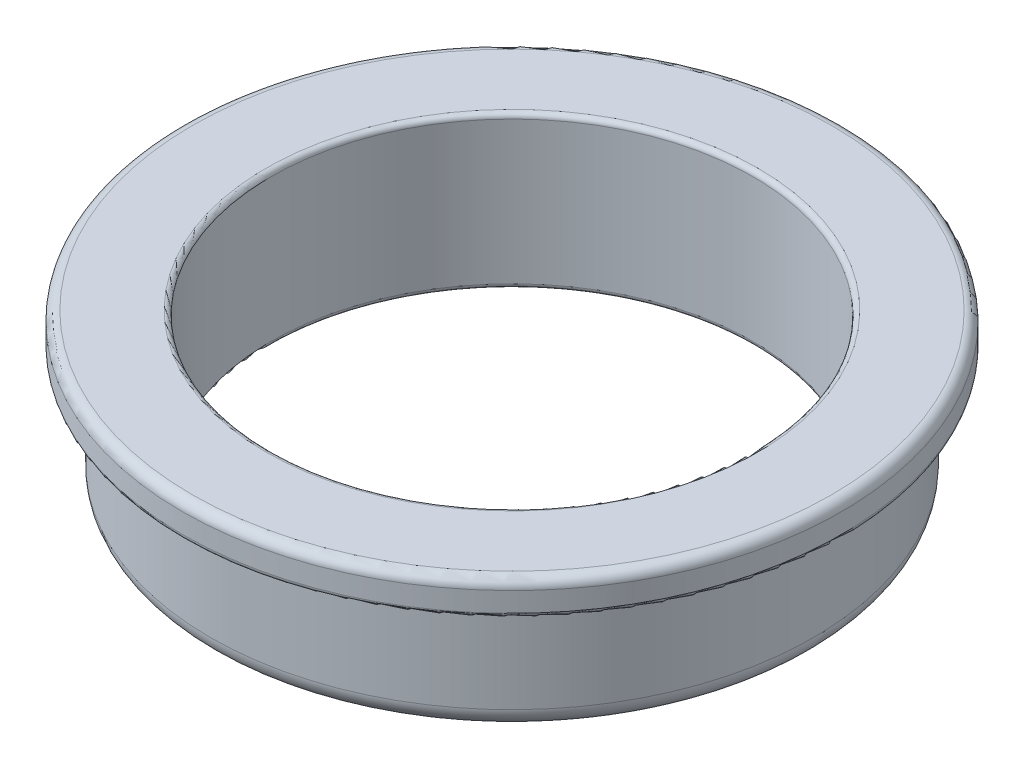
SolidWorks part; units mm, degrees
material "S45C"
ref_plane "Front Plane" through (0, 0, 0) normal (0, 0, 1) x (1, 0, 0)
ref_plane "Top Plane" through (0, 0, 0) normal (0, 1, 0) x (1, 0, 0)
ref_plane "Right Plane" through (0, 0, 0) normal (1, 0, 0) x (0, 0, -1)
sketch "Sketch1" plane through (0, 0, 0) normal (0, 1, 0) x (1, 0, 0)
  circle A0 centre (0, 0) radius 30.65
  dimension "D1" = 61.3
extrude "Boss-Extrude1" add sketch "Sketch1" against normal blind 12
sketch "Sketch2" plane through (0, 0, 0) normal (0, 1, 0) x (1, 0, 0)
  circle A0 centre (0, 0) radius 33.5
  dimension "D1" = 67
extrude "Boss-Extrude2" add sketch "Sketch2" along normal blind 3.5
sketch "Sketch3" plane through (0, 3.5, 0) normal (0, 1, 0) x (1, 0, 0)
  circle A0 centre (0, 0) radius 24.5
  dimension "D1" = 49
extrude "Cut-Extrude1" cut sketch "Sketch3" against normal through all
fillet "Fillet1" radius 1 1 edges at (0, 3.5, 33.5)
fillet "Fillet2" radius 2 1 edges at (0, -12, 30.65)
fillet "Fillet3" radius 0.5 3 edges at (0, 3.5, 24.5) (0, -12, 24.5) (0, 0, 33.5)
